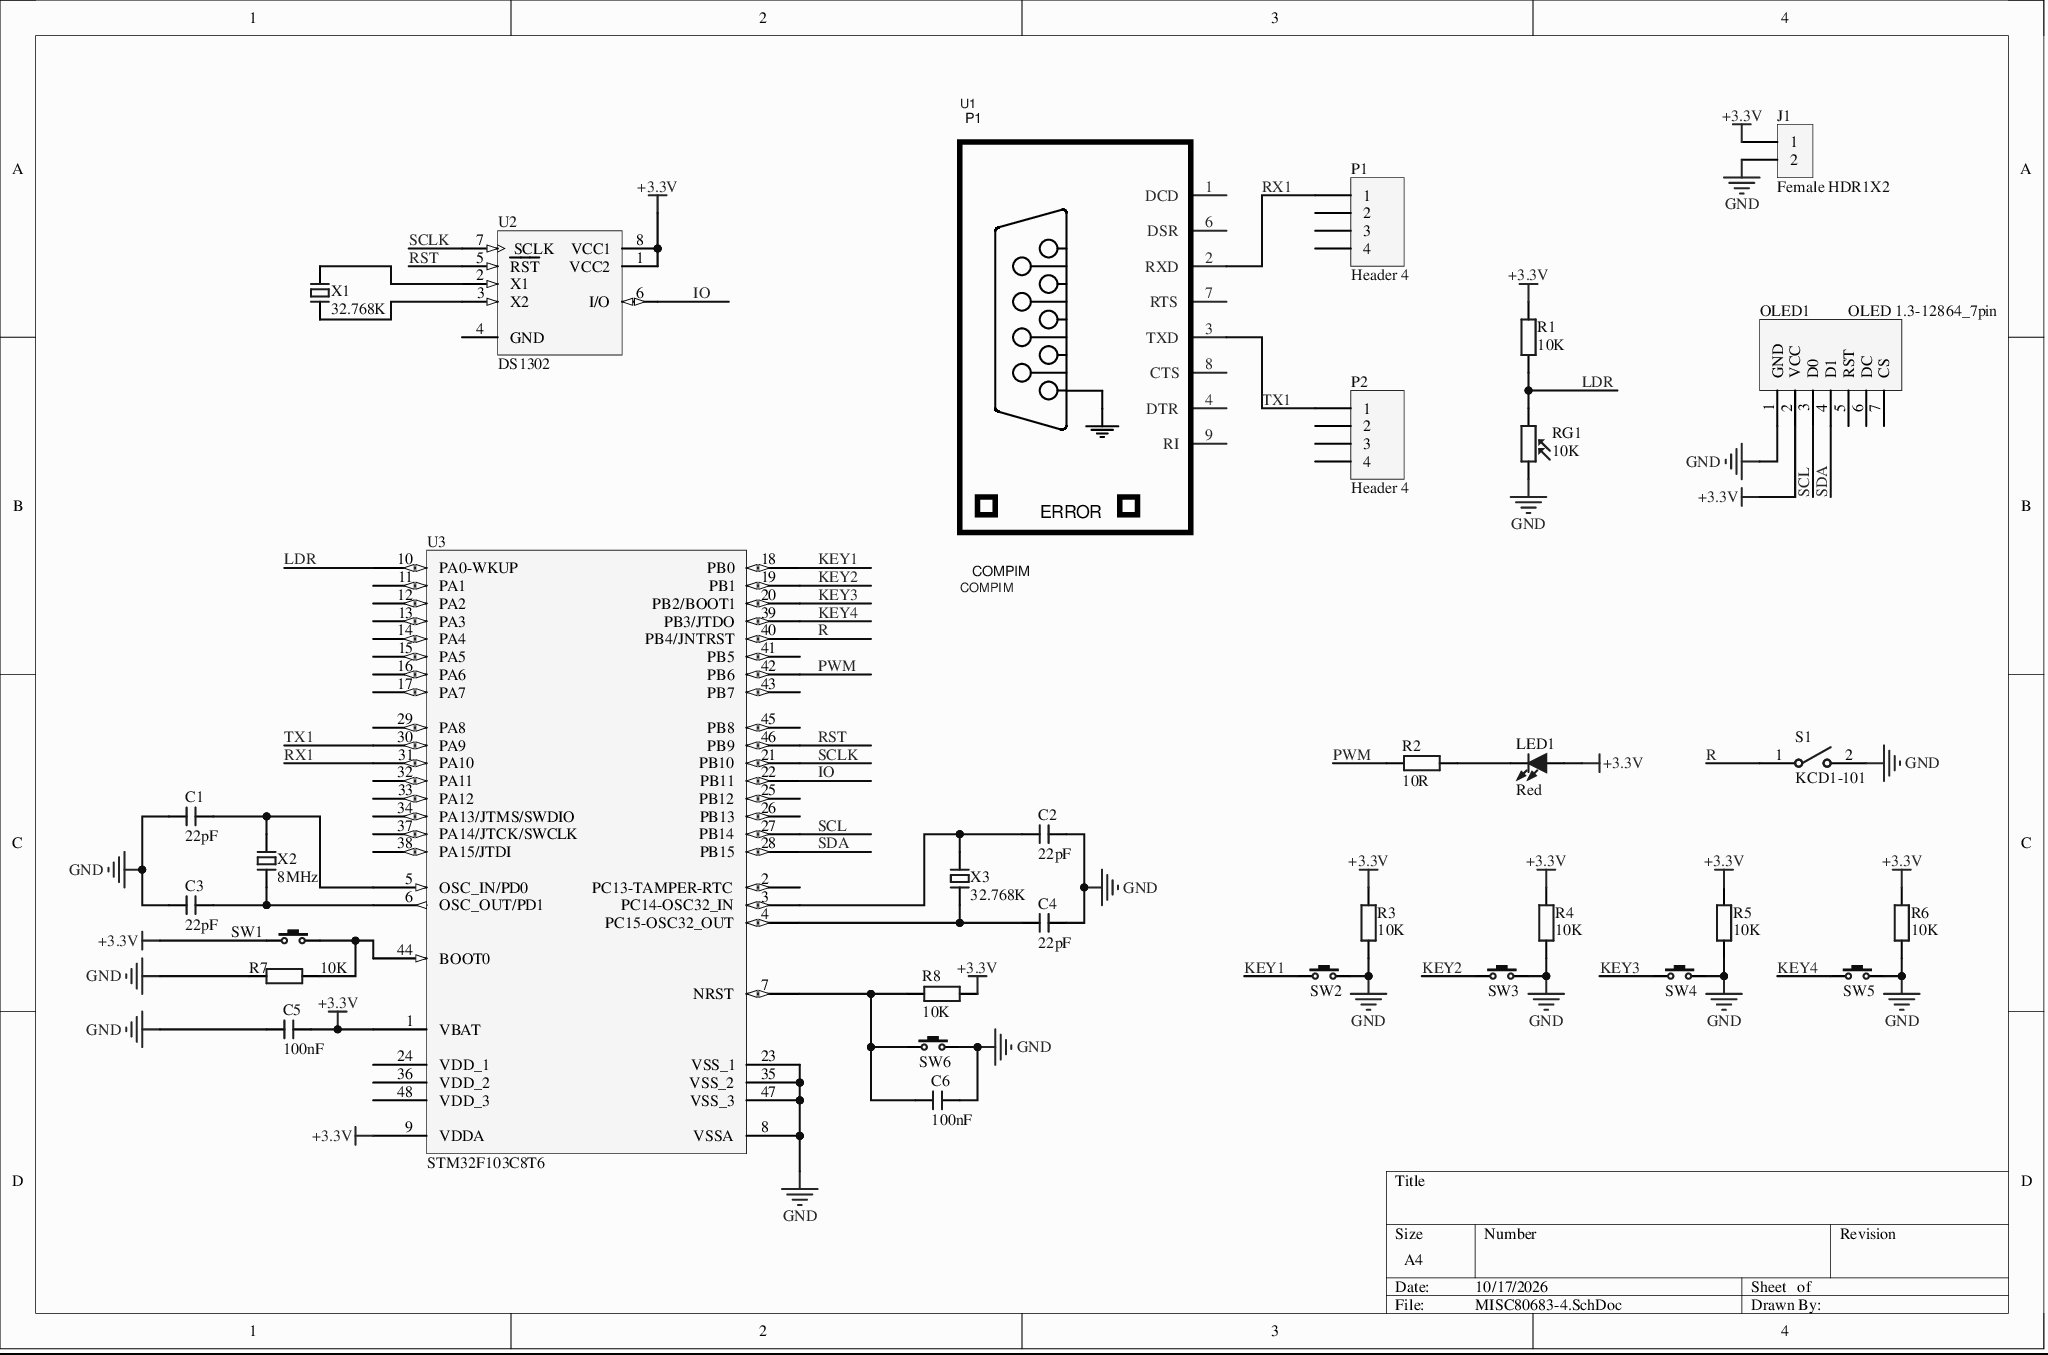
[diagram p0: MISC80683-4.SchDoc]
# Altium project MISC80683-7.PrjPcb
1 sheet, 33 parts. Net scope: global (net labels, ports and power ports of the same name join across sheets).
Board file: MISC80683.PcbDoc

## Sheet MISC80683-4.SchDoc
size A4

### Parts
C1  22pF  [C 0805_L]
C2  22pF  [C 0805_L]
C3  22pF  [C 0805_L]
C4  22pF  [C 0805_L]
C5  100nF  [C 0805_L]
C6  100nF  [C 0805_L]
J1  Female HDR1X2  [Fe-HDR1X2/2.54-S]
LED1  Red  [LED 0805G]
OLED1  OLED 1.3-12864_7pin  [OLED 1.3-12864_7pin]
P1  Header 4  [Fe-HDR1X4/2.54-S]
P2  Header 4  [Fe-HDR1X4/2.54-S]
R1  10K  [R 0805_L]
R2  10R  [R 0805_L]
R3  10K  [R 0805_L]
R4  10K  [R 0805_L]
R5  10K  [R 0805_L]
R6  10K  [R 0805_L]
R7  10K  [R 0805_L]
R8  10K  [R 0805_L]
RG1  10K  [RG5528]
S1  KCD1-101  [CSW DIP-1P]
SW1  3x6x5  [TSW SMD-3*6*2.5]  (value not drawn)
SW2  3x6x5  [TSW SMD-3*6*2.5]  (value not drawn)
SW3  3x6x5  [TSW SMD-3*6*2.5]  (value not drawn)
SW4  3x6x5  [TSW SMD-3*6*2.5]  (value not drawn)
SW5  3x6x5  [TSW SMD-3*6*2.5]  (value not drawn)
SW6  3x6x5  [TSW SMD-3*6*2.5]  (value not drawn)
U1  COMPIM  [Fe-HDR1X9/2.54-S]
U2  DS1302  [SOP8]
U3  STM32F103C8T6  [LQFP48 7X7]
X1  32.768K  [OSC 3215-2P]
X2  8MHz  [OSC 6035-2P]
X3  32.768K  [OSC 3215-2P]

### Nets
+3.3V: C5.1 J1.1 LED1.1(A) OLED1.2(VCC) R1.2 R3.2 R4.2 R5.2 R6.2 R8.2 SW1.1 U2.1(VCC2) U2.8(VCC1) U3.1(VBAT) U3.9(VDDA)
GND: C1.1 C2.2 C3.1 C4.2 C5.2 C6.2 J1.2 OLED1.1(GND) R3.1 R4.1 R5.1 R6.1 R7.1 RG1.1 S1.2 SW2.2 SW3.2 SW4.2 SW5.2 SW6.2 U3.8(VSSA) U3.23(VSS_1) U3.35(VSS_2) U3.47(VSS_3)
IO: U2.6(I/O) U3.22(PB11)
KEY1: SW2.1 U3.18(PB0)
KEY2: SW3.1 U3.19(PB1)
KEY3: SW4.1 U3.20(PB2/BOOT1)
KEY4: SW5.1 U3.39(PB3/JTDO)
LDR: R1.1 RG1.2 U3.10(PA0-WKUP)
PWM: R2.2 U3.42(PB6)
R: S1.1 U3.40(PB4/JNTRST)
RST: U2.5(~{RST}) U3.46(PB9)
RX1: P1.1 U1.2(RXD) U3.31(PA10)
SCL: OLED1.3(D0) U3.27(PB14)
SCLK: U2.7(SCLK) U3.21(PB10)
SDA: OLED1.4(D1) U3.28(PB15)
TX1: P2.1 U1.3(TXD) U3.30(PA9)
NetC1_2: C1.2 U3.5(OSC_IN/PD0) X2.2
NetC2_1: C2.1 U3.3(PC14-OSC32_IN) X3.2
NetC3_2: C3.2 U3.6(OSC_OUT/PD1) X2.1
NetC4_1: C4.1 U3.4(PC15-OSC32_OUT) X3.1
NetC6_1: C6.1 R8.1 SW6.1 U3.7(NRST)
NetLED1_2: LED1.2(K) R2.1
NetR7_2: R7.2 SW1.2 U3.44(BOOT0)
NetU2_2: U2.2(X1) X1.2
NetU2_3: U2.3(X2) X1.1

Not connected (* = marked no-connect by the designer): OLED1 5(RST)* 6(DC)* 7(CS)*; P1 2 3 4; P2 2 3 4; U1 1(DCD) 4(DTR) 6(DSR) 7(RTS) 8(CTS) 9(RI); U2 4(GND); U3 2(PC13-TAMPER-RTC) 11(PA1) 12(PA2) 13(PA3) 14(PA4) 15(PA5) 16(PA6) 17(PA7) 24(VDD_1) 25(PB12) 26(PB13) 29(PA8) 32(PA11) 33(PA12) 34(PA13/JTMS/SWDIO) 36(VDD_2) 37(PA14/JTCK/SWCLK) 38(PA15/JTDI) 41(PB5) 43(PB7) 45(PB8) 48(VDD_3)

### Library data of the parts
C1-C6 = C: Chip capacitor; BOM名称: Non-polar chip capacitor
LED1 = LED-SMD: Chip LED; BOM名称: Chip LED
OLED1 = OLED 1.3-12864_7pin: 12864 dot-matrix display; BOM名称: 12864 dot-matrix display
P1 P2 = Header 4: Header, 4-Pin; LatestRevisionDate: 17-Jul-2002; LatestRevisionNote: Re-released for DXP Platform.; Publisher: Altium Limited
R1-R8 = R: Chip resistor; BOM名称: Chip resistor
RG1 = RG: Photoresistor; BOM名称: Photoresistor
S1 = KCD1-101: 1-circuit SPST boat-type switch; BOM名称: 1-circuit SPST boat-type switch
SW1-SW6 = TSW 3x6: 3x6 tactile switch; BOM名称: 3x6 tactile switch
U2 = DS1302: Trickle Charge Timekeeping Chip; Package Information: Latest Revision: 1999; Published: 13-Oct-2000; Revision: 17-Jul-2002: Re-released for DXP Platform.; Datasheet: Latest Revision: 2-Jul-1999; Package Reference: DIP8; Publisher: Altium Limited
X1-X3 = XTAL-2P: 2-pin passive crystal; BOM名称: 2-pin passive crystal